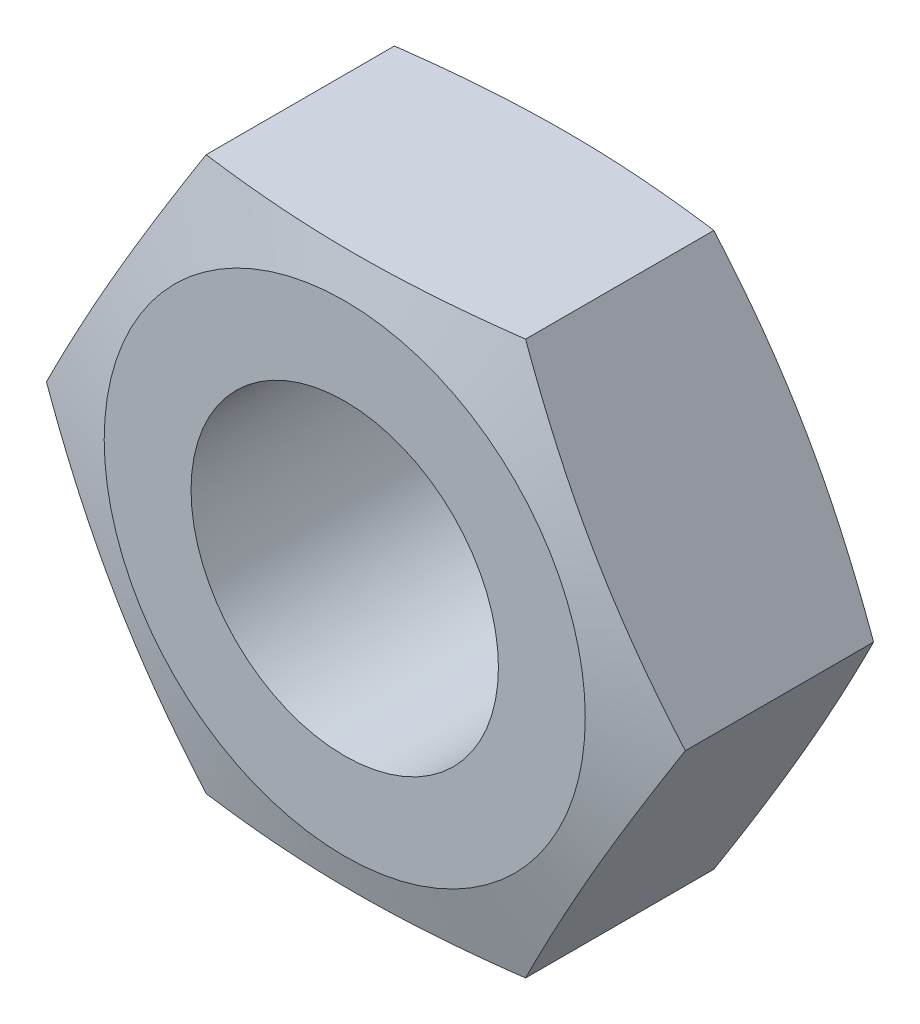
SolidWorks part; units mm, degrees
ref_plane "Front Plane" through (0, 0, 0) normal (0, 0, 1) x (1, 0, 0)
ref_plane "Top Plane" through (0, 0, 0) normal (0, 1, 0) x (1, 0, 0)
ref_plane "Right Plane" through (0, 0, 0) normal (1, 0, 0) x (0, 0, -1)
sketch "Sketch1" plane through (0, 0, 0) normal (0, 0, 1) x (1, 0, 0)
  line L2 (-20.7846, 0) -> (-10.3923, -18)
  line L3 (-10.3923, -18) -> (10.3923, -18)
  line L4 (10.3923, -18) -> (20.7846, 0)
  line L5 (20.7846, 0) -> (10.3923, 18)
  line L6 (10.3923, 18) -> (-10.3923, 18)
  line L7 (-10.3923, 18) -> (-20.7846, 0)
  circle A0 centre (0, 0) radius 10
  circle A1 centre (0, 0) radius 18 construction
  point P18 (0, 5.1962)
  dimension "D2" = 20
  dimension "D1" = 36
extrude "Boss-Extrude1" add sketch "Sketch1" along normal blind 15
cosmetic thread "Cosmetic Thread1" parameters "D2"=21
sketch "Sketch2" plane through (0, 0, 0) normal (0, 1, 0) x (1, 0, 0)
  line L0 (0, -15) -> (0, 0) construction
  line L1 (10.3923, -15) -> (-10.3923, -15) construction
  line L2 (13.7846, 0.5) -> (25.7846, -2.7154)
  line L3 (13.7846, 0.5) -> (25.7846, 0.5)
  line L4 (25.7846, 0.5) -> (25.7846, -2.7154)
  line L5 (20.7846, -15) -> (20.7846, 0) construction
  line L6 (20.7846, 0) -> (10.3923, 0) construction
  line L7 (-20.7846, -7.5) -> (20.7846, -7.5) construction
  line L8 (-20.7846, -15) -> (-20.7846, 0) construction
  line L9 (25.7846, -15.5) -> (25.7846, -12.2846)
  line L10 (13.7846, -15.5) -> (25.7846, -15.5)
  line L11 (13.7846, -15.5) -> (25.7846, -12.2846)
  dimension "D1" = 15
  dimension "D2" = 12
  dimension "D3" = 5
  dimension "D4" = 0.5
revolve "Cut-Revolve1" cut sketch "Sketch2" angle 360 about L0
